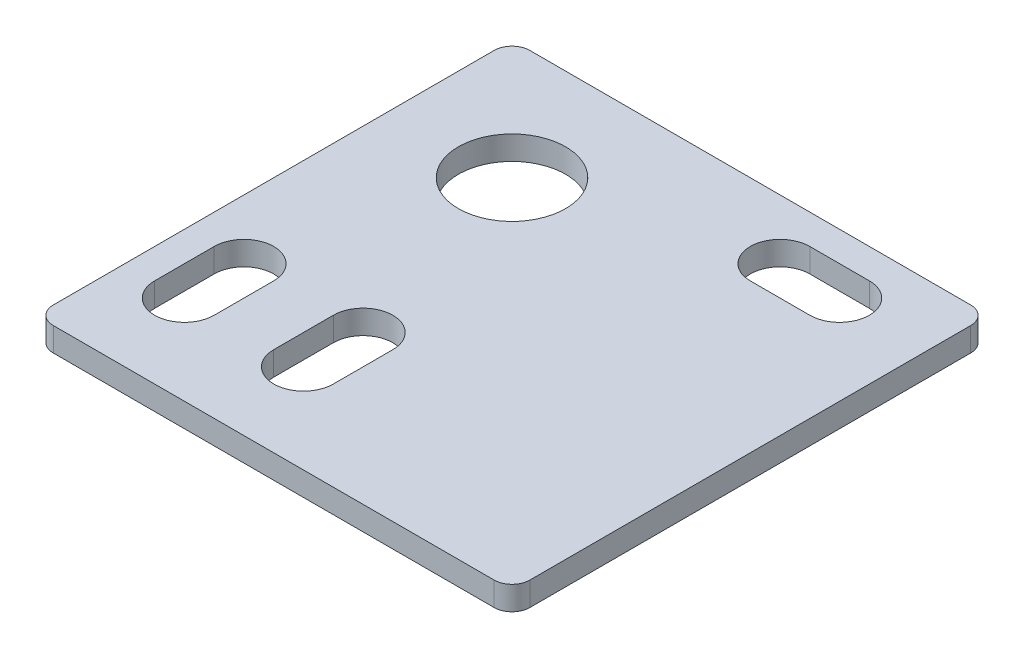
from build123d import *

# Parameters (mm, degrees)
SKETCH1_W           = 80
SKETCH1_H           = 80
SKETCH1_R           = 9
BOSS_EXTRUDE1_DEPTH = 4
FILLET1_R           = 3


with BuildPart() as part:
    # Sketch1 → Boss-Extrude1 (new body)
    with BuildSketch(Plane(origin=(0, 0, 0), x_dir=(1, 0, 0), z_dir=(0, 1, 0))):
        with Locations((-40, -40)):
            Rectangle(SKETCH1_W, SKETCH1_H)
        with Locations(Location((-60, -20, 0), (0, 0, 270))):
            Circle(SKETCH1_R, mode=Mode.SUBTRACT)
        with BuildLine():
            Line((-25, -5), (-15, -5))
            ThreePointArc((-15, -5), (-10, -10), (-15, -15))
            Line((-15, -15), (-25, -15))
            ThreePointArc((-25, -15), (-30, -10), (-25, -5))
        make_face(mode=Mode.SUBTRACT)
        with BuildLine():
            Line((-65, -55), (-65, -65))
            ThreePointArc((-65, -65), (-70, -70), (-75, -65))
            Line((-75, -65), (-75, -55))
            ThreePointArc((-75, -55), (-70, -50), (-65, -55))
        make_face(mode=Mode.SUBTRACT)
        with BuildLine():
            Line((-45, -55), (-45, -65))
            ThreePointArc((-45, -65), (-50, -70), (-55, -65))
            Line((-55, -65), (-55, -55))
            ThreePointArc((-55, -55), (-50, -50), (-45, -55))
        make_face(mode=Mode.SUBTRACT)
    extrude(amount=BOSS_EXTRUDE1_DEPTH)

    # Fillet1
    fillet1_edges = [part.edges().sort_by_distance(p)[0] for p in [
        (0, 2, 80),
        (-80, 2, 80),
        (-80, 2, 0),
        (0, 2, 0),
    ]]
    fillet(fillet1_edges, radius=FILLET1_R)


solid = part.part
